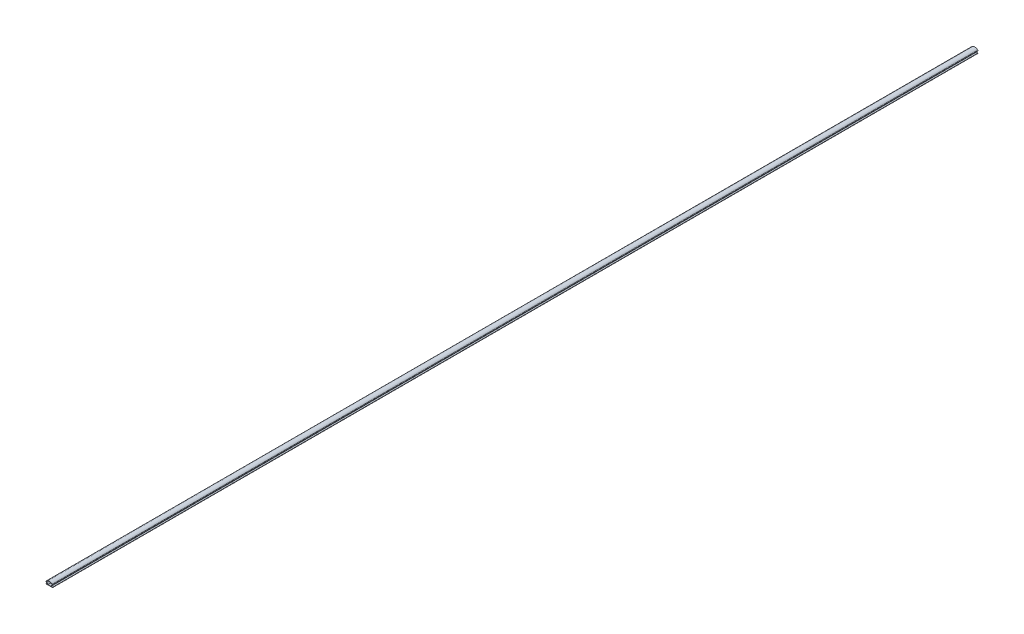
SolidWorks part; units mm, degrees
ref_plane "前视" through (0, 0, 0) normal (0, 0, 1) x (1, 0, 0)
ref_plane "上视" through (0, 0, 0) normal (0, 1, 0) x (1, 0, 0)
ref_plane "右视" through (0, 0, 0) normal (1, 0, 0) x (0, 0, -1)
sketch "草图1" plane through (0, 0, 0) normal (0, 0, 1) x (1, 0, 0)
  line L0 (0, 0) -> (0, 22.9077) construction
  line L1 (-4.5569, 4.1381) -> (-2.6457, 1.7989)
  line L2 (-2.6457, 1.7989) -> (-5, 1.7989)
  line L3 (-2, 1.7989) -> (2, 1.7989)
  line L4 (4.5569, 4.1381) -> (2.6457, 1.7989)
  line L5 (1.5915, 1.2989) -> (-5, 1.2989)
  line L6 (-4.1697, 4.4545) -> (-2, 1.7989)
  line L7 (4.1697, 4.4545) -> (2, 1.7989)
  line L8 (1.5915, 1.2989) -> (5, 1.2989)
  line L9 (-5, 1.7989) -> (-5, 1.2989)
  line L10 (5, 1.7989) -> (5, 1.2989)
  line L11 (2.6457, 1.7989) -> (5, 1.7989) construction
  line L12 (-1.5915, 1.2989) -> (-5, 1.2989) construction
  line L13 (-4.1697, 4.4545) -> (-1.5915, 1.2989) construction
  line L14 (4.1697, 4.4545) -> (1.5915, 1.2989) construction
  line L15 (2.6457, 1.7989) -> (5, 1.7989)
  arc A0 (-4.4771, 5.4902) -> (4.4771, 5.4902) centre (0, 0.8534) cw
  arc A1 (4.4771, 5.4902) -> (4.5569, 4.1381) centre (3.7825, 4.7708) cw
  arc A2 (-4.4771, 5.4902) -> (-4.5569, 4.1381) centre (-3.7825, 4.7708) ccw
  arc A3 (-4.1298, 5.1305) -> (-4.1697, 4.4545) centre (-3.7825, 4.7708) ccw
  arc A4 (-4.1298, 5.1305) -> (4.1298, 5.1305) centre (0, 0.8534) cw
  arc A5 (4.1298, 5.1305) -> (4.1697, 4.4545) centre (3.7825, 4.7708) cw
  point P12 (5.0968, 4.7989)
  point P15 (-5.0968, 4.7989)
  dimension "D4" = 1
  dimension "D1" = 10
  dimension "D2" = 5.5
  dimension "D3" = 3
  dimension "D6" = 4
  dimension "D5" = 0.5
extrude "凸台-拉伸1" add sketch "草图1" along normal mid plane 1410
